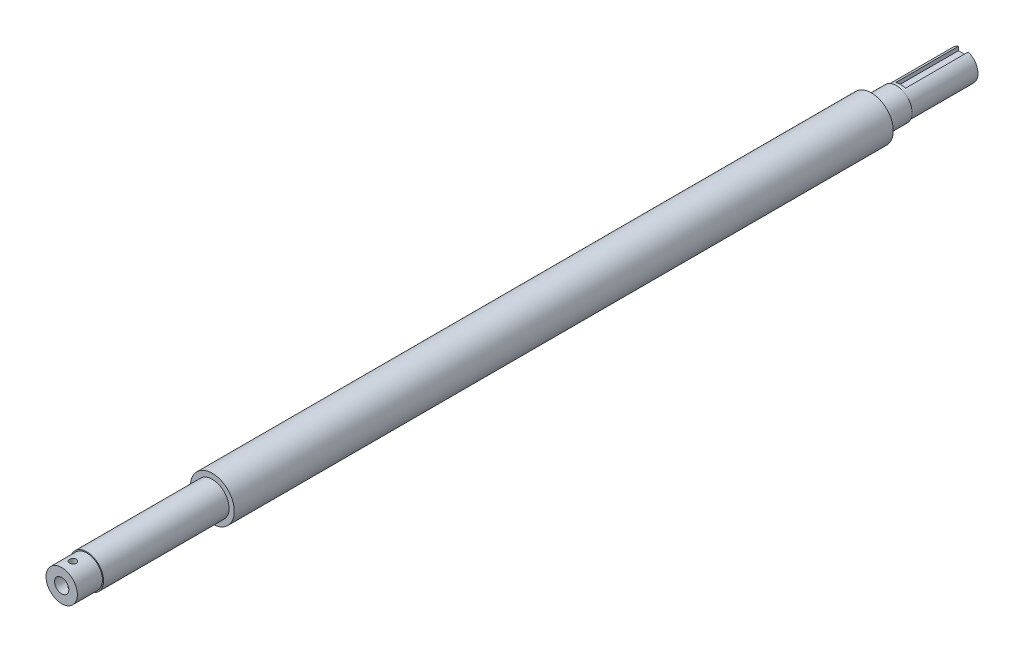
from build123d import *

# Parameters (mm, degrees)
SKETCH_1_R             = 7.5
EXTRUDE_1_DEPTH        = 12
SKETCH_2_R             = 8
EXTRUDE_2_DEPTH        = 60
SKETCH_3_R             = 10.5
EXTRUDE_3_DEPTH        = 315
EXTRUDE_START          = 12
SKETCH_4_R             = 7.5
EXTRUDE_4_DEPTH        = 12
SKETCH_5_R             = 7
EXTRUDE_5_DEPTH        = 32
SKETCH_6_W             = 4.707373346
SKETCH_6_H             = 4.483082856
CUT_EXTRUDE_1_DEPTH    = 30
HOLE_WIZARD_M8_1_D     = 6.8
HOLE_WIZARD_M8_1_DEPTH = 19.75
HOLE_WIZARD_M8_1_TIP   = 2.042926105
HOLE_WIZARD_M4_1_D     = 3.3


with BuildPart() as part:
    # 草图1 → 凸台-拉伸1 (new body)
    with BuildSketch(Plane.XY):
        Circle(SKETCH_1_R)
    extrude(amount=EXTRUDE_1_DEPTH)

    # 草图2 → 凸台-拉伸2 (add)
    with BuildSketch(Plane(origin=(0, 0, 0), x_dir=(-1, 0, 0), z_dir=(0, 0, -1))):
        Circle(SKETCH_2_R)
    extrude(amount=EXTRUDE_2_DEPTH)

    # 草图3 → 凸台-拉伸3 (add)
    with BuildSketch(Plane(origin=(0, 0, -60), x_dir=(-1, 0, 0), z_dir=(0, 0, -1))):
        Circle(SKETCH_3_R)
    extrude(amount=EXTRUDE_3_DEPTH)

    # 草图4 → 凸台-拉伸4 (add)
    with BuildSketch(Plane(origin=(0, 0, -375), x_dir=(-1, 0, 0), z_dir=(0, 0, -1)).offset(EXTRUDE_START)):
        Circle(SKETCH_4_R)
    extrude(amount=-EXTRUDE_4_DEPTH)

    # 草图5 → 凸台-拉伸5 (add)
    with BuildSketch(Plane(origin=(0, 0, -387), x_dir=(-1, 0, 0), z_dir=(0, 0, -1))):
        Circle(SKETCH_5_R)
    extrude(amount=EXTRUDE_5_DEPTH)

    # 草图6 → 切除-拉伸1 (cut)
    with BuildSketch(Plane(origin=(0, 0, -419), x_dir=(-1, 0, 0), z_dir=(0, 0, -1))):
        with Locations((0, 7)):
            Rectangle(SKETCH_6_W, SKETCH_6_H)
    extrude(amount=-CUT_EXTRUDE_1_DEPTH, mode=Mode.SUBTRACT)

    # M8 螺纹孔1
    with Locations(Plane.XY.offset(12)):
        with Locations((0, 0)):
            Hole(HOLE_WIZARD_M8_1_D / 2, depth=HOLE_WIZARD_M8_1_DEPTH)
            with Locations((0, 0, -(HOLE_WIZARD_M8_1_DEPTH + HOLE_WIZARD_M8_1_TIP / 2))):  # 118° drill point
                Cone(0, HOLE_WIZARD_M8_1_D / 2, HOLE_WIZARD_M8_1_TIP, mode=Mode.SUBTRACT)

    # M4 螺纹孔1 (through all)
    with Locations(Plane(origin=(-0.010980736, 7.499991962, 6.6634249), x_dir=(0.999998928208, 0.001464098146, 0), z_dir=(-0.001464098146, 0.999998928208, 0))):
        with Locations((0, 0)):
            Hole(HOLE_WIZARD_M4_1_D / 2)


solid = part.part
